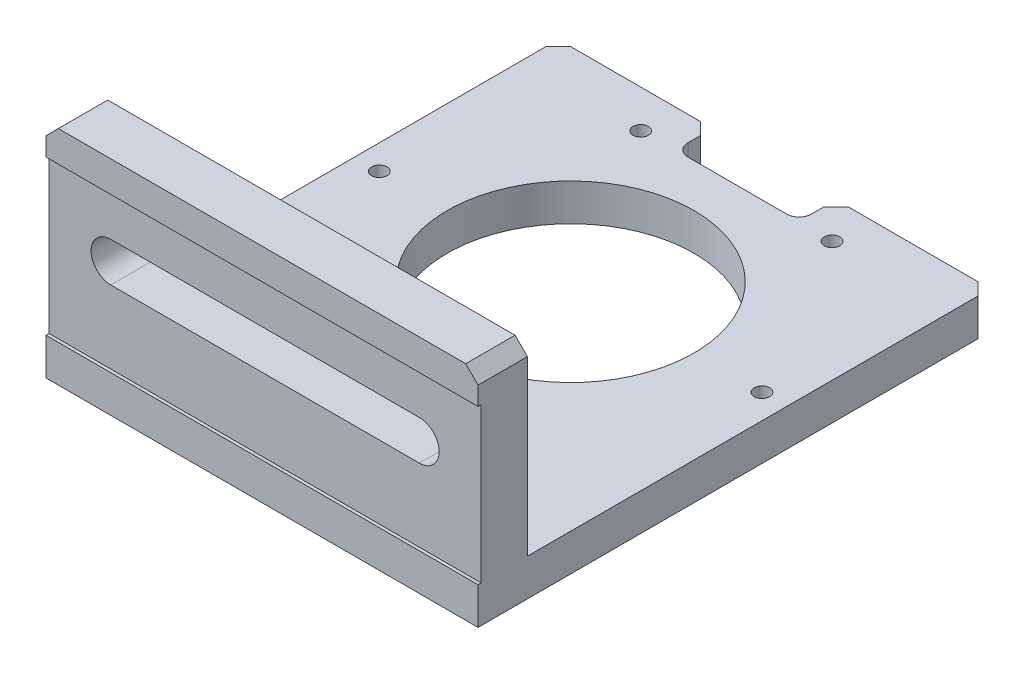
from build123d import *

# Parameters (mm, degrees)
SKETCH1_W           = 70
SKETCH1_H           = 83
BOSS_EXTRUDE1_DEPTH = 6
SKETCH2_W           = 70
SKETCH2_H           = 8
BOSS_EXTRUDE2_DEPTH = 30
SKETCH3_R           = 20
CUT_EXTRUDE1_DEPTH  = 20
SKETCH4_W           = 20
SKETCH4_H           = 12.019208042
CUT_EXTRUDE2_DEPTH  = 20
SKETCH5_R           = 1.25
CUT_EXTRUDE3_DEPTH  = 20
CUT_EXTRUDE4_DEPTH  = 20
SKETCH7_W           = 0.5
SKETCH7_H           = 25
CUT_EXTRUDE5_DEPTH  = 90
FILLET1_R           = 2
CHAMFER1_SIZE       = 2


with BuildPart() as part:
    # Sketch1 → Boss-Extrude1 (new body)
    with BuildSketch(Plane(origin=(0, 0, 0), x_dir=(1, 0, 0), z_dir=(0, 1, 0))):
        Rectangle(SKETCH1_W, SKETCH1_H)
    extrude(amount=BOSS_EXTRUDE1_DEPTH)

    # Sketch2 → Boss-Extrude2 (add)
    with BuildSketch(Plane(origin=(0, 6, 0), x_dir=(1, 0, 0), z_dir=(0, 1, 0))):
        with Locations((0, -37.5)):
            Rectangle(SKETCH2_W, SKETCH2_H)
    extrude(amount=BOSS_EXTRUDE2_DEPTH)

    # Sketch3 → Cut-Extrude1 (cut)
    with BuildSketch(Plane.XZ):
        with Locations(Location((0, -8.5, 0), (0, 0, 270))):
            Circle(SKETCH3_R)
    extrude(amount=-CUT_EXTRUDE1_DEPTH, mode=Mode.SUBTRACT)

    # Sketch4 → Cut-Extrude2 (cut)
    with BuildSketch(Plane(origin=(0, 6, 0), x_dir=(1, 0, 0), z_dir=(0, 1, 0))):
        with Locations((0, 41.509604021)):
            Rectangle(SKETCH4_W, SKETCH4_H)
    extrude(amount=-CUT_EXTRUDE2_DEPTH, mode=Mode.SUBTRACT)

    # Sketch5 → Cut-Extrude3 (cut)
    with BuildSketch(Plane(origin=(0, 6, 0), x_dir=(1, 0, 0), z_dir=(0, 1, 0))):
        with Locations(Location((31, 8.5, 0), (0, 0, 270))):
            Circle(SKETCH5_R)
        with Locations(Location((15.5, -18.346787517, 0), (0, 0, 270))):
            Circle(SKETCH5_R)
        with Locations(Location((-15.5, -18.346787517, 0), (0, 0, 270))):
            Circle(SKETCH5_R)
        with Locations(Location((-31, 8.5, 0), (0, 0, 270))):
            Circle(SKETCH5_R)
        with Locations(Location((-15.5, 35.346787517, 0), (0, 0, 270))):
            Circle(SKETCH5_R)
        with Locations(Location((15.5, 35.346787517, 0), (0, 0, 270))):
            Circle(SKETCH5_R)
    extrude(amount=-CUT_EXTRUDE3_DEPTH, mode=Mode.SUBTRACT)

    # Sketch6 → Cut-Extrude4 (cut)
    with BuildSketch(Plane(origin=(0, 0, 33.5), x_dir=(-1, 0, 0), z_dir=(0, 0, -1))):
        with BuildLine():
            Line((25, 17.8), (-25, 17.8))
            ThreePointArc((-25, 17.8), (-28.2, 21), (-25, 24.2))
            Line((-25, 24.2), (25, 24.2))
            ThreePointArc((25, 24.2), (28.2, 21), (25, 17.8))
        make_face()
    extrude(amount=-CUT_EXTRUDE4_DEPTH, mode=Mode.SUBTRACT)

    # Sketch7 → Cut-Extrude5 (cut)
    with BuildSketch(Plane.ZY.offset(35)):
        with Locations((41.25, 18.5)):
            Rectangle(SKETCH7_W, SKETCH7_H)
    extrude(amount=-CUT_EXTRUDE5_DEPTH, mode=Mode.SUBTRACT)

    # Fillet1
    fillet1_edges = [part.edges().sort_by_distance(p)[0] for p in [
        (-10, 3, -35.5),
        (10, 3, -35.5),
    ]]
    fillet(fillet1_edges, radius=FILLET1_R)

    # Chamfer1
    chamfer1_edges = [part.edges().sort_by_distance(p)[0] for p in [
        (-35, 36, 37.5),
        (35, 36, 37.5),
        (-10, 3, -41.5),
        (10, 3, -41.5),
        (-35, 3, -41.5),
        (35, 3, -41.5),
    ]]
    chamfer(chamfer1_edges, length=CHAMFER1_SIZE)


solid = part.part
